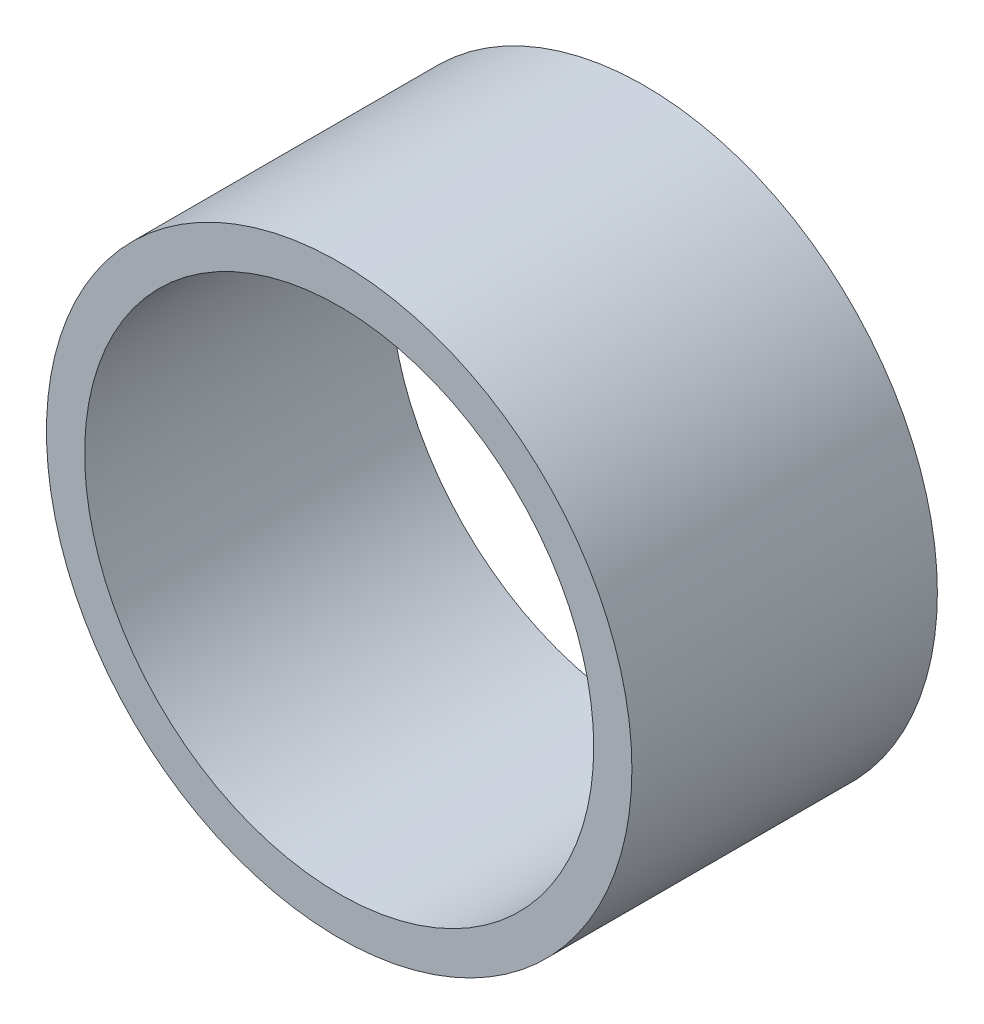
SolidWorks part; units mm, degrees
material "Q235"
ref_plane "Front Plane" through (0, 0, 0) normal (0, 0, 1) x (1, 0, 0)
ref_plane "Top Plane" through (0, 0, 0) normal (0, 1, 0) x (1, 0, 0)
ref_plane "Right Plane" through (0, 0, 0) normal (1, 0, 0) x (0, 0, -1)
sketch "Sketch1" plane through (0, 0, 0) normal (0, 0, 1) x (1, 0, 0)
  circle A0 centre (0, 0) radius 11.5
  circle A1 centre (0, 0) radius 10
  dimension "D1" = 20
  dimension "D2" = 23
extrude "Boss-Extrude1" add sketch "Sketch1" along normal blind 12
